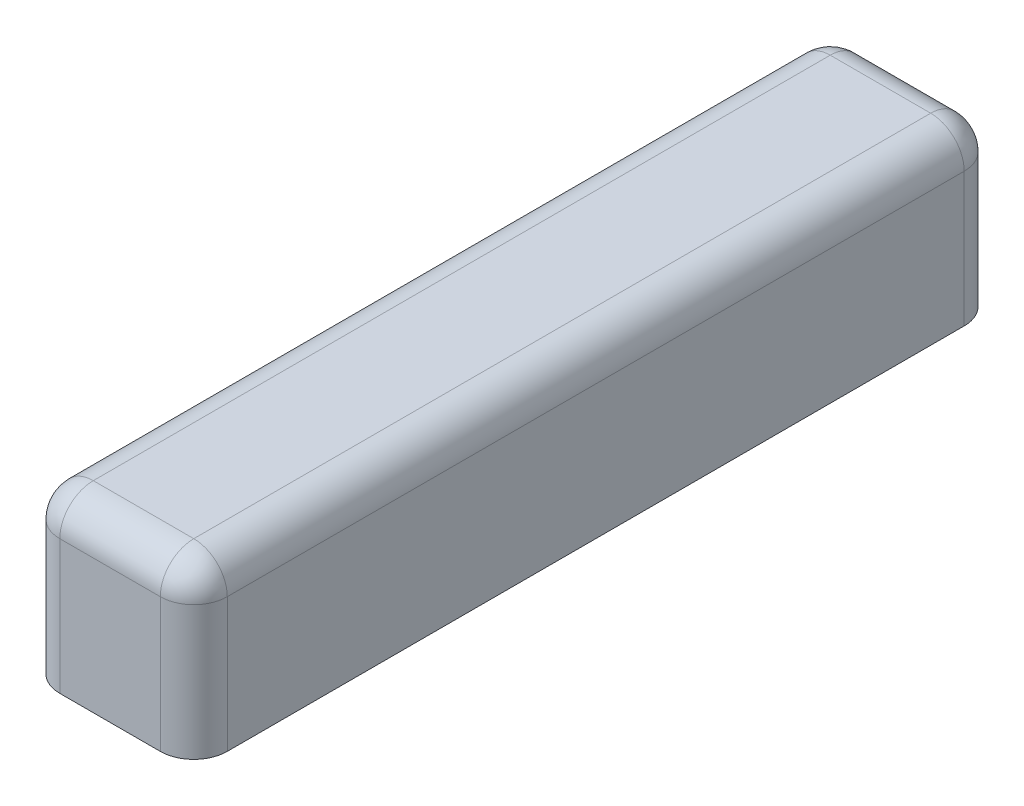
SolidWorks part; units mm, degrees
material "橡胶"
ref_plane "前视基准面" through (0, 0, 0) normal (0, 0, 1) x (1, 0, 0)
ref_plane "上视基准面" through (0, 0, 0) normal (0, 1, 0) x (1, 0, 0)
ref_plane "右视基准面" through (0, 0, 0) normal (1, 0, 0) x (0, 0, -1)
sketch "草图1" plane through (0, 0, 0) normal (0, 0, 1) x (1, 0, 0)
  line L0 (0, 0) -> (50, 0)
  line L1 (50, 0) -> (50, 50)
  line L2 (50, 50) -> (0, 50)
  line L3 (0, 0) -> (0, 50)
extrude "凸台-拉伸2" add sketch "草图1" along normal blind 240
sketch "草图2" plane through (0, 0, 0) normal (0, -1, 0) x (1, 0, 0)
  line L0 (0, 240) -> (0, 290)
  line L1 (0, 290) -> (50, 290)
  line L2 (50, 290) -> (50, 0)
  line L3 (50, 0) -> (50, -50)
  line L4 (50, -50) -> (0, -50)
  line L5 (0, -50) -> (0, 240)
extrude "凸台-拉伸3" add sketch "草图2" along normal blind 5
fillet "圆角1" radius 10 8 edges at (25, 50, 240) (50, 50, 120) (25, 50, 0) (0, 50, 120)
sketch "草图3" plane through (0, 0, 0) normal (-1, 0, 0) x (0, 0, 1)
  line L0 (-50, 0) -> (-50, -5)
  line L1 (-50, -5) -> (290, -5)
  line L2 (290, -5) -> (290, 0)
  line L3 (290, 0) -> (-50, 0)
extrude "切除-拉伸1" cut sketch "草图3" against normal blind 59
